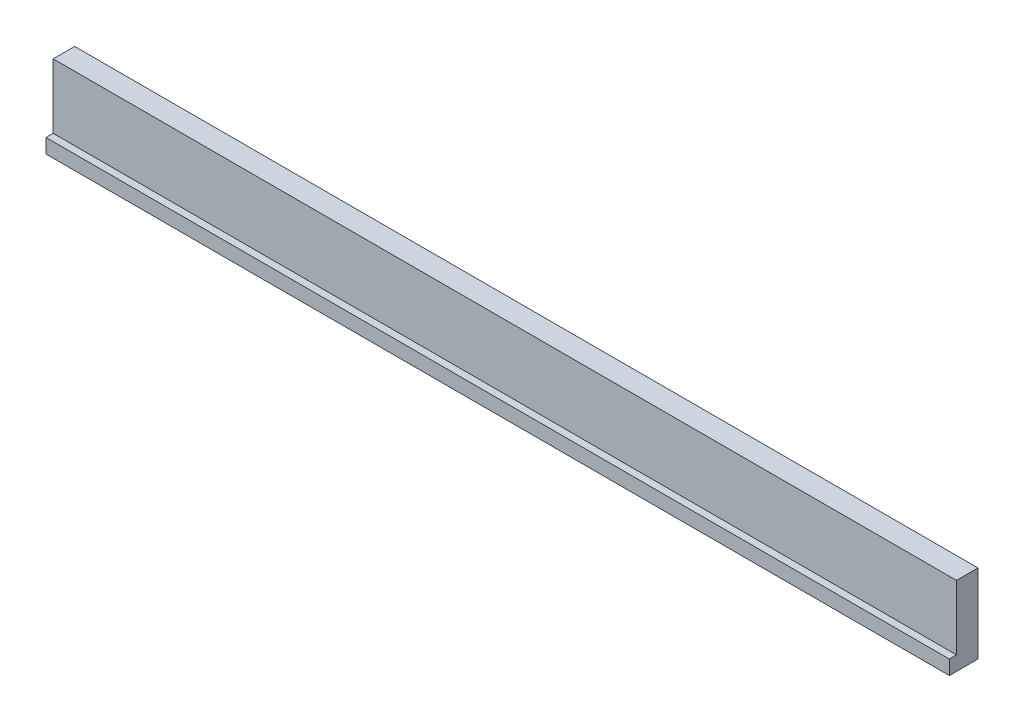
SolidWorks part; units mm, degrees
ref_plane "Front Plane" through (0, 0, 0) normal (0, 0, 1) x (1, 0, 0)
ref_plane "Top Plane" through (0, 0, 0) normal (0, 1, 0) x (1, 0, 0)
ref_plane "Right Plane" through (0, 0, 0) normal (1, 0, 0) x (0, 0, -1)
sketch "Sketch1" plane through (0, 0, 0) normal (1, 0, 0) x (0, 0, -1)
  line L0 (-31.2155, 48.1086) -> (-31.2155, -6.8914)
  line L1 (-51.2155, -6.8914) -> (-31.2155, -6.8914)
  line L7 (-46.2155, 48.1086) -> (-46.2155, 3.1086)
  line L8 (-51.2155, 3.1086) -> (-46.2155, 3.1086)
  line L9 (-51.2155, -6.8914) -> (-51.2155, 3.1086)
  line L10 (-31.2155, 48.1086) -> (-46.2155, 48.1086)
extrude "Boss-Extrude1" add sketch "Sketch1" against normal blind 630
